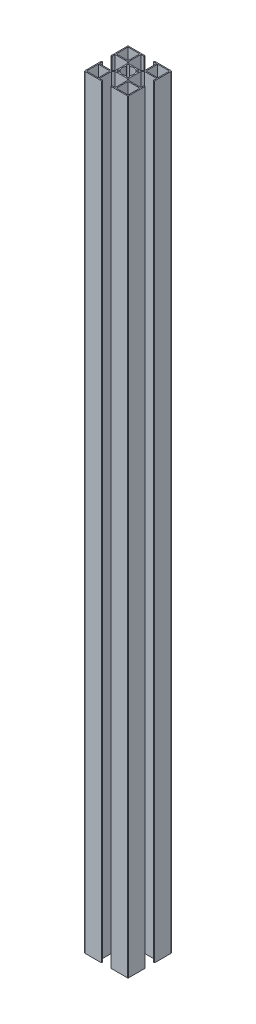
from build123d import *

# Parameters (mm, degrees)
SKETCH1_W               = 10.85
SKETCH1_H               = 10.85
BOSS_EXTRUDE1_DEPTH     = 700
MIRROR2_COPY_1_SKETCH_W = 10.85
MIRROR2_COPY_1_SKETCH_H = 10.85
MIRROR2_COPY_1_DEPTH    = 700


with BuildPart() as part:
    # Sketch1 → Boss-Extrude1 (new body)
    with BuildSketch(Plane(origin=(0, 0, 0), x_dir=(1, 0, 0), z_dir=(0, 1, 0))):
        with BuildLine():
            Line((-4.3, 20), (-19.5, 20))
            ThreePointArc((-19.5, 20), (-19.853553391, 19.853553391), (-20, 19.5))
            Line((-20, 19.5), (-20, 4.3))
            Line((-20, 4.3), (-19.05, 4.3))
            Line((-19.05, 4.3), (-19.05, 7.25))
            Line((-19.05, 7.25), (-7.921751442, 7.25))
            Line((-7.921751442, 7.25), (-6.2, 5.528248558))
            Line((-6.2, 5.528248558), (-6.2, 0))
            Line((-6.2, 0), (-5.3, 0))
            ThreePointArc((-5.3, 0), (-5.066731596, 1.555066215), (-4.387460025, 2.973246463))
            Line((-4.387460025, 2.973246463), (-5.091168825, 3.676955262))
            ThreePointArc((-5.091168825, 3.676955262), (-5.091168825, 5.091168825), (-3.676955262, 5.091168825))
            Line((-3.676955262, 5.091168825), (-2.973246463, 4.387460025))
            ThreePointArc((-2.973246463, 4.387460025), (-1.555066215, 5.066731596), (0, 5.3))
            Line((0, 5.3), (0, 6.2))
            Line((0, 6.2), (-5.528248558, 6.2))
            Line((-5.528248558, 6.2), (-7.25, 7.921751442))
            Line((-7.25, 7.921751442), (-7.25, 19.05))
            Line((-7.25, 19.05), (-4.3, 19.05))
            Line((-4.3, 19.05), (-4.3, 20))
        make_face()
        with Locations((-13.625, 13.625)):
            Rectangle(SKETCH1_W, SKETCH1_H, mode=Mode.SUBTRACT)
    boss_extrude1 = extrude(amount=BOSS_EXTRUDE1_DEPTH)

    # Mirror1: Boss-Extrude1 across plane
    add(boss_extrude1.mirror(Plane(origin=(0, 0, 0), x_dir=(0, 0, 1), z_dir=(1, 0, 0))))

    # Mirror2: Boss-Extrude1 across plane
    add(boss_extrude1.mirror(Plane.XY))

    # Mirror2 copy 1 sketch → Mirror2 copy 1 (add)
    with BuildSketch(Plane(origin=(0, 0, 0), x_dir=(-1, 0, 0), z_dir=(0, 1, 0))):
        with BuildLine():
            Line((-4.3, 20), (-19.5, 20))
            ThreePointArc((-19.5, 20), (-19.853553391, 19.853553391), (-20, 19.5))
            Line((-20, 19.5), (-20, 4.3))
            Line((-20, 4.3), (-19.05, 4.3))
            Line((-19.05, 4.3), (-19.05, 7.25))
            Line((-19.05, 7.25), (-7.921751442, 7.25))
            Line((-7.921751442, 7.25), (-6.2, 5.528248558))
            Line((-6.2, 5.528248558), (-6.2, 0))
            Line((-6.2, 0), (-5.3, 0))
            ThreePointArc((-5.3, 0), (-5.066731596, 1.555066215), (-4.387460025, 2.973246463))
            Line((-4.387460025, 2.973246463), (-5.091168825, 3.676955262))
            ThreePointArc((-5.091168825, 3.676955262), (-5.091168825, 5.091168825), (-3.676955262, 5.091168825))
            Line((-3.676955262, 5.091168825), (-2.973246463, 4.387460025))
            ThreePointArc((-2.973246463, 4.387460025), (-1.555066215, 5.066731596), (0, 5.3))
            Line((0, 5.3), (0, 6.2))
            Line((0, 6.2), (-5.528248558, 6.2))
            Line((-5.528248558, 6.2), (-7.25, 7.921751442))
            Line((-7.25, 7.921751442), (-7.25, 19.05))
            Line((-7.25, 19.05), (-4.3, 19.05))
            Line((-4.3, 19.05), (-4.3, 20))
        make_face()
        with Locations((-13.625, 13.625)):
            Rectangle(MIRROR2_COPY_1_SKETCH_W, MIRROR2_COPY_1_SKETCH_H, mode=Mode.SUBTRACT)
    extrude(amount=MIRROR2_COPY_1_DEPTH)


solid = part.part
